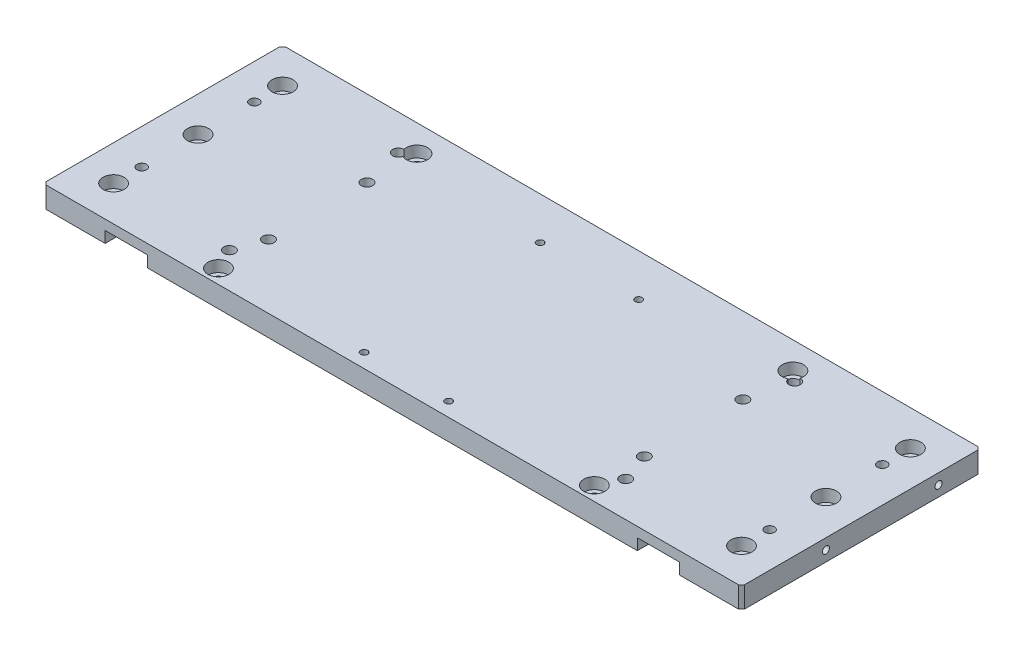
SolidWorks part; units mm, degrees
ref_plane "Front Plane" through (0, 0, 0) normal (0, 0, 1) x (1, 0, 0)
ref_plane "Top Plane" through (0, 0, 0) normal (0, 1, 0) x (1, 0, 0)
ref_plane "Right Plane" through (0, 0, 0) normal (1, 0, 0) x (0, 0, -1)
sketch "Sketch1" plane through (0, 0, 0) normal (0, 1, 0) x (1, 0, 0)
  line L1 (248, -85) -> (-248, -85)
  line L2 (248, -85) -> (248, 85)
  line L3 (248, 85) -> (-248, 85)
  line L4 (-248, -85) -> (-248, 85)
  line L5 (248, -85) -> (-248, 85) construction
  line L6 (248, 85) -> (-248, -85) construction
  point P0 (0, 0)
  dimension "D1" = 496
  dimension "D2" = 170
extrude "Boss-Extrude1" add sketch "Sketch1" along normal blind 15
hole_wizard "CBORE for M8 Hex Socket Head Cap Screw2" positions "Sketch3" profile "Sketch2" counterbore size "M8" standard "Iso"
sketch "Sketch3" plane through (0, 15, 0) normal (0, 1, 0) x (-1, 0, 0)
  line L4 (248, -85) -> (248, 85) construction
  line L5 (-248, 0) -> (248, 0) construction
  line L6 (-248, 85) -> (-248, -85) construction
  point P0 (223, -60)
  point P1 (223, 0)
  point P3 (223, 60)
  dimension "D1" = 120
  dimension "D2" = 25
sketch "Sketch2" plane through (-223, 15, -60) normal (1, 0, 0) x (0, 0, 1)
  line L0 (0, 0) -> (0, 15)
  line L1 (0, 15) -> (4.5, 15)
  line L3 (4.5, 15) -> (4.5, 8.6)
  line L4 (4.5, 8.6) -> (7.5, 8.6)
  line L5 (7.5, 8.6) -> (7.5, 0)
  line L7 (7.5, 0) -> (0, 0)
  line L11 (0, -6.35) -> (0, 107.95) construction
  dimension "通孔孔直径" = 9
  dimension "通孔孔深度" = 15
  dimension "柱形沉头孔直径" = 15
  dimension "柱形沉头孔深度" = 8.6
sketch "Sketch4" plane through (0, 0, 0) normal (0, -1, 0) x (1, 0, 0)
  line L1 (140.75, -60) -> (-140.75, -60) construction
  line L2 (140.75, -60) -> (140.75, 60) construction
  line L3 (140.75, 60) -> (-140.75, 60) construction
  line L4 (-140.75, -60) -> (-140.75, 60) construction
  line L5 (140.75, -60) -> (-140.75, 60) construction
  line L6 (140.75, 60) -> (-140.75, -60) construction
  circle A0 centre (140.75, 60) radius 4
  circle A1 centre (140.75, -60) radius 4
  circle A2 centre (-140.75, -60) radius 4
  circle A3 centre (-140.75, 60) radius 4
  point P8 (0, 0)
  dimension "D3" = 8
  dimension "D1" = 120
  dimension "D2" = 281.5
extrude "Cut-Extrude1" cut sketch "Sketch4" against normal through all
sketch "Sketch5" plane through (0, 0, 0) normal (0, -1, 0) x (1, 0, 0)
  line L2 (133.5, -30.5) -> (133.5, 39.5) construction
  line L4 (-133.5, -30.5) -> (-133.5, 39.5) construction
  circle A0 centre (133.5, -30.5) radius 4
  circle A1 centre (133.5, 39.5) radius 4
  circle A2 centre (-133.5, 39.5) radius 4
  circle A3 centre (-133.5, -30.5) radius 4
  dimension "D4" = 8
extrude "Cut-Extrude2" cut sketch "Sketch5" against normal through all
hole_wizard "CBORE for M8 Hex Socket Head Cap Screw1" positions "Sketch7" profile "Sketch6" counterbore size "M8" standard "Iso"
sketch "Sketch7" plane through (0, 15, 0) normal (0, 1, 0) x (-1, 0, 0)
  point P0 (133.5, -66)
  point P1 (-133.5, -66)
  point P3 (133.5, 75)
  point P5 (-133.5, 75)
sketch "Sketch6" plane through (-133.5, 15, -66) normal (1, 0, 0) x (0, 0, 1)
  line L0 (0, 0) -> (0, 15)
  line L1 (0, 15) -> (4.5, 15)
  line L3 (4.5, 15) -> (4.5, 8)
  line L4 (4.5, 8) -> (7.5, 8)
  line L5 (7.5, 8) -> (7.5, 0)
  line L7 (7.5, 0) -> (0, 0)
  line L11 (0, -6.35) -> (0, 107.95) construction
  dimension "通孔孔直径" = 9
  dimension "通孔孔深度" = 15
  dimension "柱形沉头孔直径" = 15
  dimension "柱形沉头孔深度" = 8
hole_wizard "M6 Tapped Hole1" positions "Sketch9" profile "Sketch8" tap size "M6" standard "ISO"
sketch "Sketch9" plane through (248, 0, 0) normal (1, 0, 0) x (0, 0, -1)
  line L0 (-85, 0) -> (85, 0) construction
  line L1 (85, 15) -> (85, 0) construction
  point P0 (55, 7.5)
  point P1 (-25, 7.5)
  dimension "D1" = 7.5
  dimension "D2" = 30
  dimension "D3" = 80
sketch "Sketch8" plane through (248, 7.5, -55) normal (0, 1, 0) x (0, 0, -1)
  line L0 (0, 0) -> (0, 16.5022)
  line L1 (0, 16.5022) -> (2.5, 15)
  line L2 (2.5, 15) -> (2.5, 0)
  line L5 (2.5, 0) -> (0, 0)
  line L10 (0, 16.5022) -> (-2.5, 15) construction
  line L11 (0, -6.35) -> (0, 107.95) construction
  dimension "螺纹孔钻头直径" = 5
  dimension "螺纹孔钻头深度" = 15
  dimension "导头角度" = 118
cosmetic thread "Cosmetic Thread1" parameters "D1"=12, "D2"=6
cosmetic thread "Cosmetic Thread2" parameters "D1"=12, "D2"=6
hole_wizard "M6 Tapped Hole2" positions "Sketch11" profile "Sketch10" tap size "M6" standard "ISO"
sketch "Sketch11" plane through (0, 0, 0) normal (0, -1, 0) x (1, 0, 0)
  line L0 (248, -85) -> (-248, -85) construction
  point P0 (-35, -55)
  point P1 (35, -55)
  dimension "D1" = 35
  dimension "D2" = 35
  dimension "D3" = 30
  dimension "D4" = 30
sketch "Sketch10" plane through (-35, 0, -55) normal (1, 0, 0) x (0, 0, -1)
  line L0 (0, 0) -> (0, 15)
  line L1 (0, 15) -> (2.5, 15)
  line L2 (2.5, 15) -> (2.5, 0)
  line L5 (2.5, 0) -> (0, 0)
  line L11 (0, -6.35) -> (0, 107.95) construction
  dimension "通孔螺纹孔钻头直径" = 5
  dimension "通孔螺纹孔钻头深度" = 15
cosmetic thread "Cosmetic Thread3" parameters "D2"=6
cosmetic thread "Cosmetic Thread4" parameters "D2"=6
chamfer "Chamfer1" distance 2 angle 45
hole_wizard "M6 Tapped Hole3" positions "Sketch13" profile "Sketch12" tap size "M6" standard "ISO"
sketch "Sketch13" plane through (0, 0, 0) normal (0, -1, 0) x (1, 0, 0)
  line L0 (-246, 85) -> (246, 85) construction
  point P0 (-30, 75)
  point P1 (30, 75)
  dimension "D1" = 30
  dimension "D2" = 30
  dimension "D3" = 10
  dimension "D4" = 10
sketch "Sketch12" plane through (-30, 0, 75) normal (1, 0, 0) x (0, 0, -1)
  line L0 (0, 0) -> (0, 15)
  line L1 (0, 15) -> (2.5, 15)
  line L2 (2.5, 15) -> (2.5, 0)
  line L5 (2.5, 0) -> (0, 0)
  line L11 (0, -6.35) -> (0, 107.95) construction
  dimension "通孔螺纹孔钻头直径" = 5
  dimension "通孔螺纹孔钻头深度" = 15
cosmetic thread "Cosmetic Thread5" parameters "D2"=6
cosmetic thread "Cosmetic Thread14" parameters "D2"=6
hole_wizard "M6 Tapped Hole4" positions "Sketch15" profile "Sketch14" tap size "M6" standard "ISO"
sketch "Sketch15" plane through (0, 0, -85) normal (0, 0, -1) x (-1, 0, 0)
  line L0 (-246, 0) -> (246, 0) construction
  point P0 (0, 7.5)
  point P1 (100, 7.5)
  point P3 (-100, 7.5)
  dimension "D1" = 7.5
  dimension "D2" = 100
  dimension "D3" = 100
sketch "Sketch14" plane through (0, 7.5, -85) normal (1, 0, 0) x (0, 1, 0)
  line L0 (0, 0) -> (0, 16.5022)
  line L1 (0, 16.5022) -> (2.5, 15)
  line L2 (2.5, 15) -> (2.5, 0)
  line L5 (2.5, 0) -> (0, 0)
  line L10 (0, 16.5022) -> (-2.5, 15) construction
  line L11 (0, -6.35) -> (0, 107.95) construction
  dimension "螺纹孔钻头直径" = 5
  dimension "螺纹孔钻头深度" = 15
  dimension "导头角度" = 118
cosmetic thread "Cosmetic Thread7" parameters "D1"=12, "D2"=6
cosmetic thread "Cosmetic Thread8" parameters "D1"=12, "D2"=6
cosmetic thread "Cosmetic Thread9" parameters "D1"=12, "D2"=6
mirror "Mirror1" about plane through (0, 0, 0) normal (1, 0, 0) of "CBORE for M8 Hex Socket Head Cap Screw2"
hole_wizard "M8 Tapped Hole1" positions "Sketch17" profile "Sketch16" tap size "M8" standard "Iso"
sketch "Sketch17" plane through (0, 0, 0) normal (0, -1, 0) x (1, 0, 0)
  point P0 (-223, 40)
  point P2 (-223, -40)
  point P5 (223, -40)
  point P8 (223, 40)
sketch "Sketch16" plane through (-223, 0, 40) normal (1, 0, 0) x (0, 0, -1)
  line L0 (0, 0) -> (0, 15)
  line L1 (0, 15) -> (3.4, 15)
  line L2 (3.4, 15) -> (3.4, 0)
  line L5 (3.4, 0) -> (0, 0)
  line L11 (0, -6.35) -> (0, 107.95) construction
  dimension "通孔螺纹孔钻头直径" = 6.8
  dimension "通孔螺纹孔钻头深度" = 15
cosmetic thread "Cosmetic Thread10" parameters "D2"=8
cosmetic thread "Cosmetic Thread11" parameters "D2"=8
cosmetic thread "Cosmetic Thread12" parameters "D2"=8
cosmetic thread "Cosmetic Thread13" parameters "D2"=8
sketch "Sketch18" plane through (0, 0, 0) normal (0, -1, 0) x (1, 0, 0)
  line L0 (-246, 85) -> (246, 85) construction
  line L1 (-204, 85) -> (-174, 85)
  line L2 (-204, 85) -> (-204, -85)
  line L3 (-204, -85) -> (-174, -85)
  line L4 (-174, 85) -> (-174, -85)
  line L5 (246, -85) -> (-246, -85) construction
  line L6 (-248, -83) -> (-248, 83) construction
  line L7 (0, 0) -> (0, -85) construction
  line L8 (204, 85) -> (204, -85)
  line L9 (204, 85) -> (174, 85)
  line L10 (204, -85) -> (174, -85)
  line L11 (174, 85) -> (174, -85)
  dimension "D1" = 30
  dimension "D2" = 44
extrude "Cut-Extrude3" cut sketch "Sketch18" against normal blind 8
